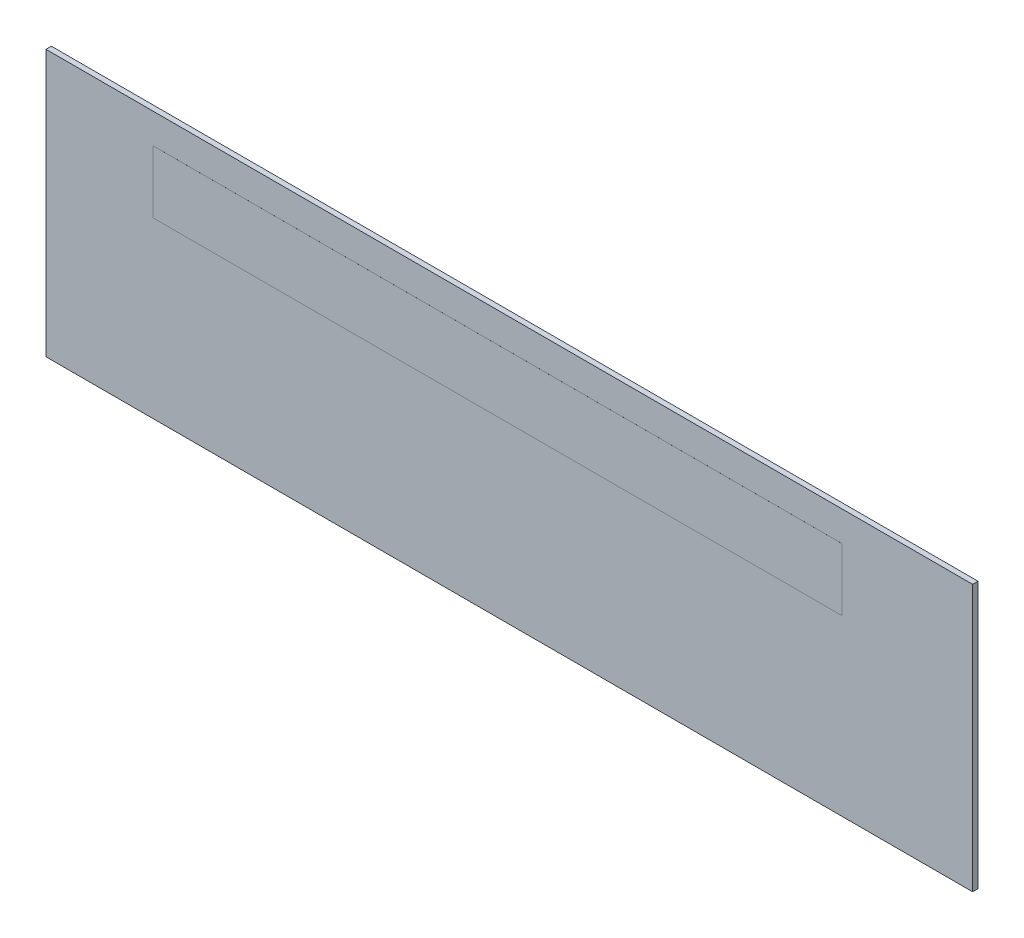
from build123d import *

# Parameters (mm, degrees)
SKETCH1_W           = 515
SKETCH1_H           = 148
BOSS_EXTRUDE1_DEPTH = 3
SKETCH2_W           = 382.967454029
SKETCH2_H           = 34.69619669
BOSS_EXTRUDE2_DEPTH = 0.01


with BuildPart() as part:
    # Sketch1 → Boss-Extrude1 (new body)
    with BuildSketch(Plane.XY):
        Rectangle(SKETCH1_W, SKETCH1_H)
    extrude(amount=BOSS_EXTRUDE1_DEPTH)

    # Sketch2 → Boss-Extrude2 (add)
    with BuildSketch(Plane.XY.offset(3)):
        with Locations((-6.627399213, 39.979630289)):
            Rectangle(SKETCH2_W, SKETCH2_H)
    extrude(amount=BOSS_EXTRUDE2_DEPTH)


solid = part.part
